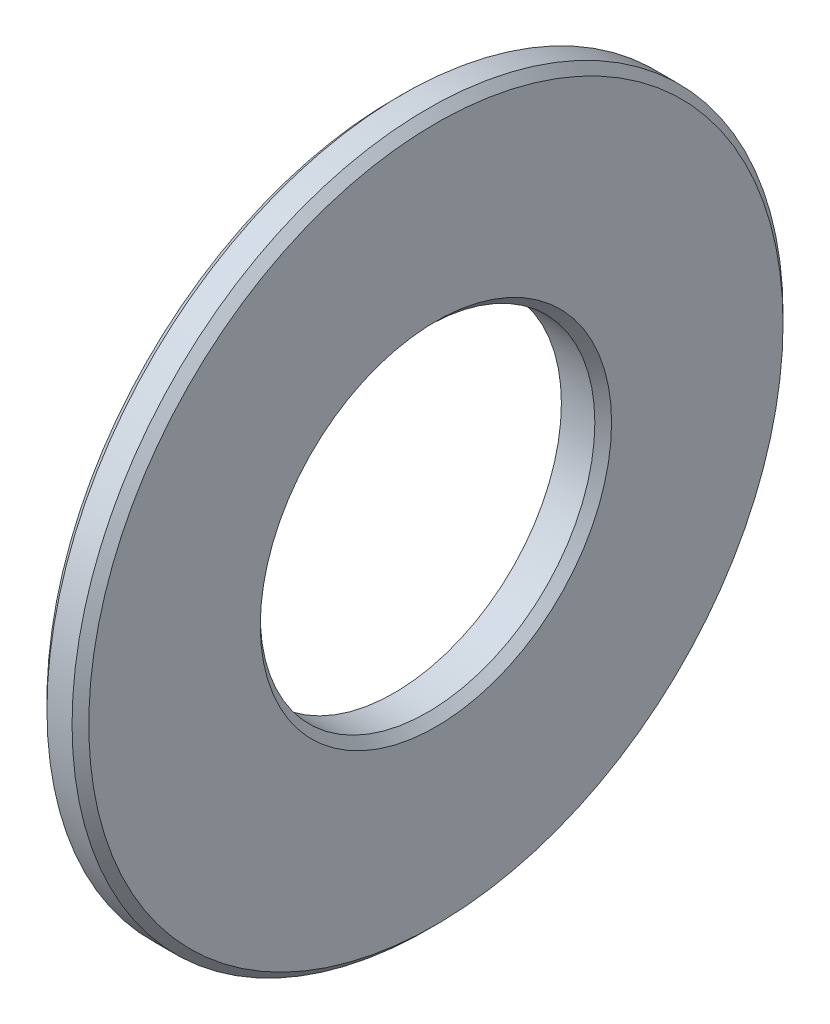
from build123d import *

# Parameters (mm, degrees)
SKETCH1_R           = 85
SKETCH1_R_2         = 40
BOSS_EXTRUDE1_DEPTH = 10
CHAMFER1_SIZE       = 2


with BuildPart() as part:
    # Sketch1 → Boss-Extrude1 (new body)
    with BuildSketch(Plane(origin=(0, 0, 0), x_dir=(0, 0, -1), z_dir=(1, 0, 0))):
        Circle(SKETCH1_R)
        Circle(SKETCH1_R_2, mode=Mode.SUBTRACT)
    extrude(amount=BOSS_EXTRUDE1_DEPTH)

    # Chamfer1
    chamfer1_edges = [part.edges().sort_by_distance(p)[0] for p in [
        (0, 0, 85),
        (10, 0, 85),
        (10, 0, 40),
    ]]
    chamfer(chamfer1_edges, length=CHAMFER1_SIZE)


solid = part.part
